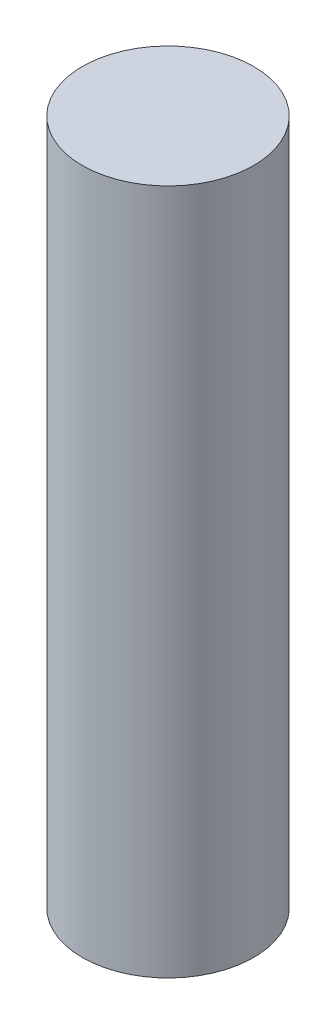
from build123d import *

# Parameters (mm, degrees)
SKETCH1_R           = 12.5
BOSS_EXTRUDE1_DEPTH = 100


with BuildPart() as part:
    # Sketch1 → Boss-Extrude1 (new body)
    with BuildSketch(Plane(origin=(0, 0, 0), x_dir=(1, 0, 0), z_dir=(0, 1, 0))):
        with Locations(Location((0, 0, 0), (0, 0, 90))):
            Circle(SKETCH1_R)
    extrude(amount=BOSS_EXTRUDE1_DEPTH)


solid = part.part
